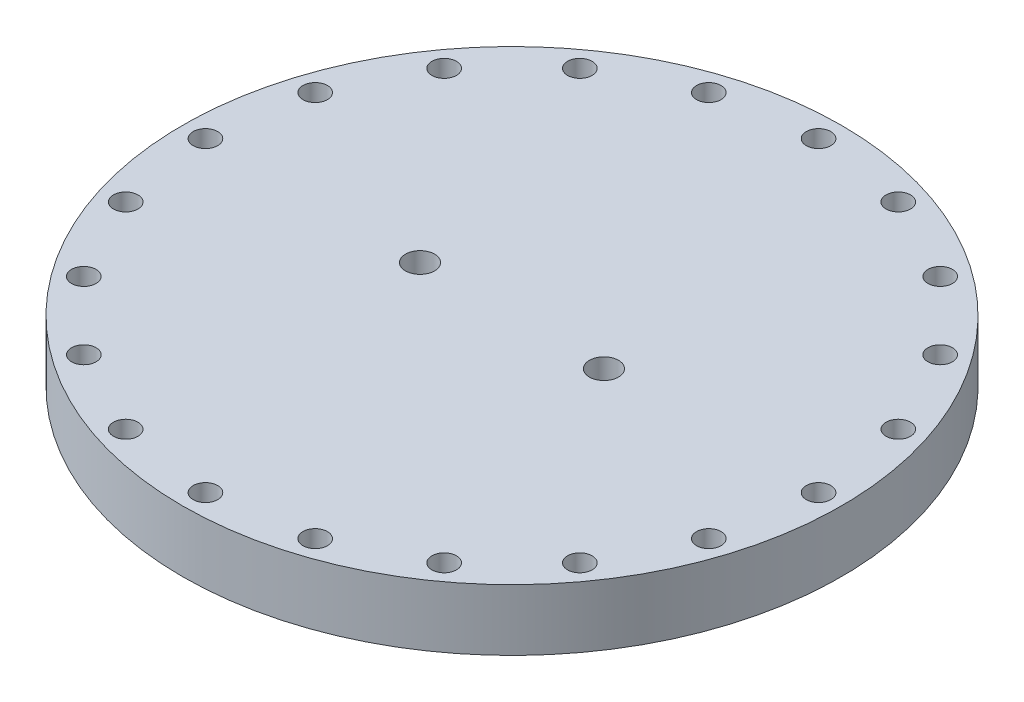
from build123d import *

# Parameters (mm, degrees)
SKETCH1_R                  = 215
BOSS_EXTRUDE1_DEPTH        = 40
F_16_0_16_DIAMETER_HOLE1_D = 16
G1_2_TAPPED_HOLE1_D        = 19


with BuildPart() as part:
    # Sketch1 → Boss-Extrude1 (new body)
    with BuildSketch(Plane(origin=(0, 0, 0), x_dir=(1, 0, 0), z_dir=(0, 1, 0))):
        with Locations(Location((0, 0, 0), (0, 0, 270))):
            Circle(SKETCH1_R)
    extrude(amount=BOSS_EXTRUDE1_DEPTH)

    # Ø16.0 (16) Diameter Hole1 (through all)
    with Locations(Plane(origin=(0, 40, 0), x_dir=(1, 0, 0), z_dir=(0, 1, 0))):
        with Locations((200, 0), (190.211303259, -61.803398875), (161.803398875, -117.557050458), (117.557050458, -161.803398875), (61.803398875, -190.211303259), (0, -200), (-61.803398875, -190.211303259), (-117.557050458, -161.803398875), (-161.803398875, -117.557050458), (-190.211303259, -61.803398875), (-200, 0), (-190.211303259, 61.803398875), (-161.803398875, 117.557050458), (-117.557050458, 161.803398875), (-61.803398875, 190.211303259), (0, 200), (61.803398875, 190.211303259), (117.557050458, 161.803398875), (161.803398875, 117.557050458), (190.211303259, 61.803398875)):
            Hole(F_16_0_16_DIAMETER_HOLE1_D / 2)

    # G1/2 Tapped Hole1 (through all)
    with Locations(Plane(origin=(0, 40, 0), x_dir=(1, 0, 0), z_dir=(0, 1, 0))):
        with Locations((-60, 0), (60, 0)):
            Hole(G1_2_TAPPED_HOLE1_D / 2)


solid = part.part
